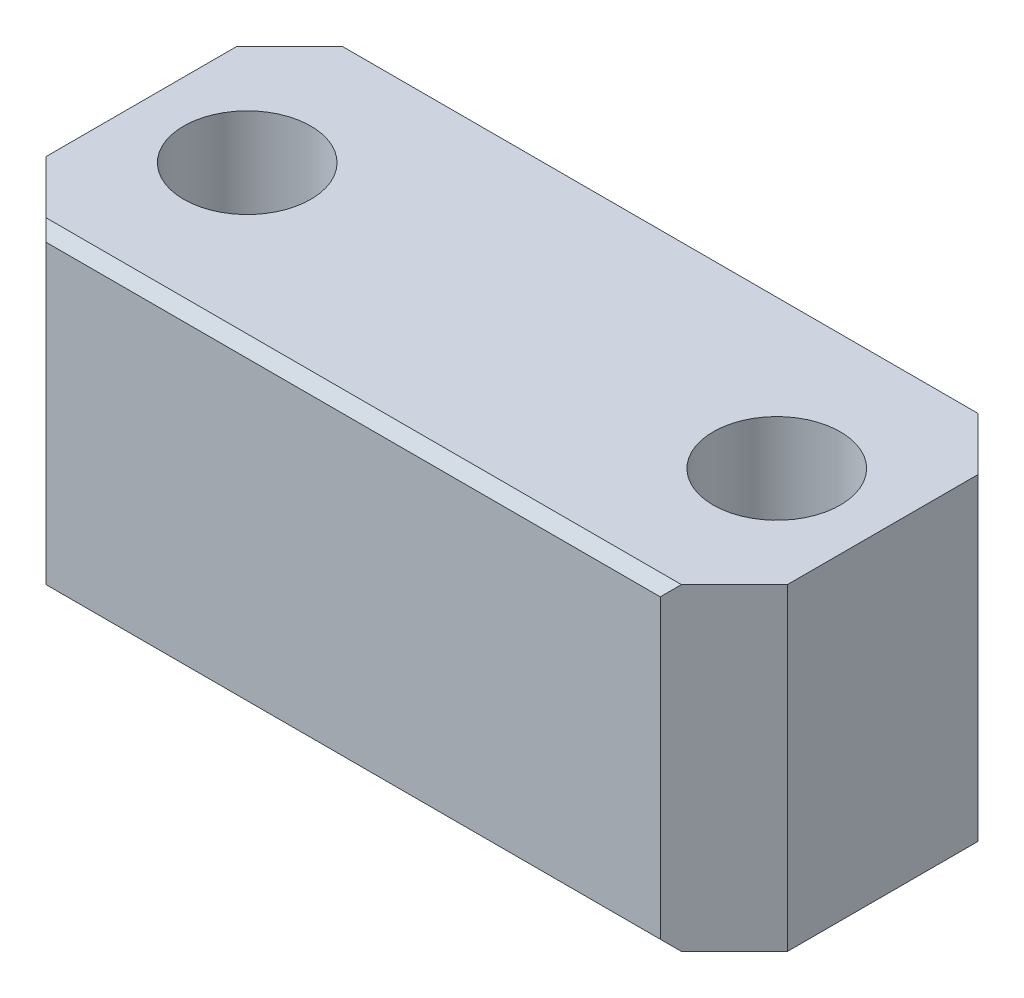
from build123d import *

# Parameters (mm, degrees)
SKETCH1_W           = 35
SKETCH1_H           = 15
BOSS_EXTRUDE1_DEPTH = 15
SKETCH2_R           = 3
CUT_EXTRUDE1_DEPTH  = 15.7
CHAMFER1_SIZE       = 3
CHAMFER2_SIZE       = 0.5


with BuildPart() as part:
    # Sketch1 → Boss-Extrude1 (new body)
    with BuildSketch(Plane(origin=(0, 0, 0), x_dir=(1, 0, 0), z_dir=(0, 1, 0))):
        with Locations((-67.573325782, 9.634846385)):
            Rectangle(SKETCH1_W, SKETCH1_H)
    extrude(amount=BOSS_EXTRUDE1_DEPTH)

    # Sketch2 → Cut-Extrude1 (cut)
    with BuildSketch(Plane(origin=(0, 15, 0), x_dir=(1, 0, 0), z_dir=(0, 1, 0))):
        with Locations(Location((-80.073325782, 9.634846385, 0), (0, 0, 270))):
            Circle(SKETCH2_R)
        with Locations(Location((-55.073325782, 9.634846385, 0), (0, 0, 270))):
            Circle(SKETCH2_R)
    extrude(amount=-CUT_EXTRUDE1_DEPTH, mode=Mode.SUBTRACT)

    # Chamfer1
    chamfer1_edges = [part.edges().sort_by_distance(p)[0] for p in [
        (-85.073325782, 7.5, -17.134846385),
        (-50.073325782, 7.5, -17.134846385),
        (-50.073325782, 7.5, -2.134846385),
        (-85.073325782, 7.5, -2.134846385),
    ]]
    chamfer(chamfer1_edges, length=CHAMFER1_SIZE)

    # Chamfer2
    chamfer2_edges = [part.edges().sort_by_distance(p)[0] for p in [
        (-67.573325782, 0, -17.134846385),
        (-67.573325782, 0, -2.134846385),
        (-67.573325782, 15, -2.134846385),
        (-67.573325782, 15, -17.134846385),
    ]]
    chamfer(chamfer2_edges, length=CHAMFER2_SIZE)


solid = part.part
